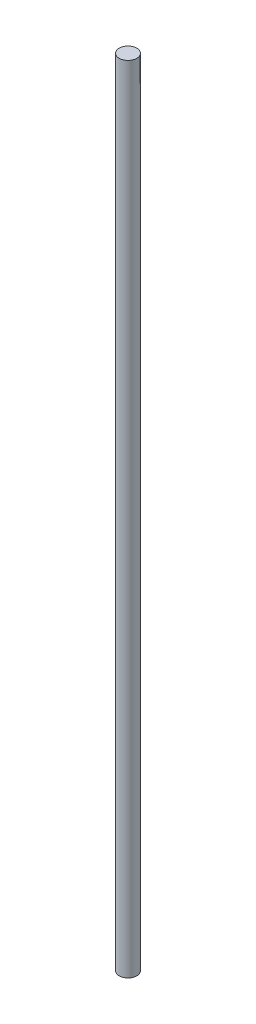
SolidWorks part; units mm, degrees
ref_plane "前视基准面" through (0, 0, 0) normal (0, 0, 1) x (1, 0, 0)
ref_plane "上视基准面" through (0, 0, 0) normal (0, 1, 0) x (1, 0, 0)
ref_plane "右视基准面" through (0, 0, 0) normal (1, 0, 0) x (0, 0, -1)
sketch "草图1" plane through (0, 0, 0) normal (0, 1, 0) x (1, 0, 0)
  circle A0 centre (0, 0) radius 2
  dimension "D1" = 4
extrude "凸台-拉伸1" add sketch "草图1" along normal blind 180
